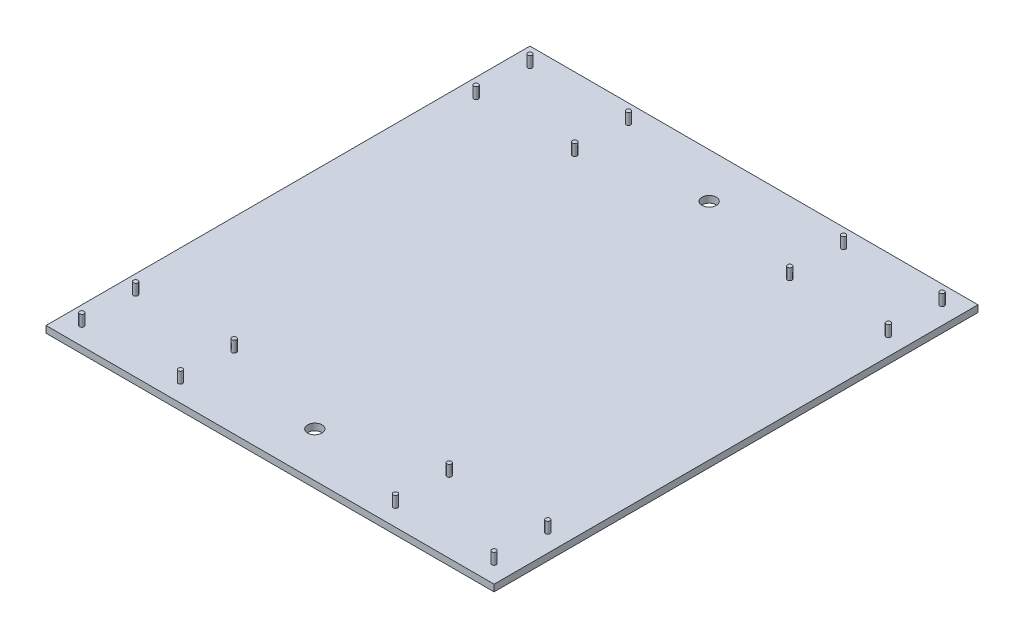
from build123d import *

# Parameters (mm, degrees)
SKETCH1_W           = 2000
SKETCH1_H           = 2160
BOSS_EXTRUDE1_DEPTH = 30
SKETCH2_R           = 10
BOSS_EXTRUDE2_DEPTH = 50
SKETCH3_R           = 32
CUT_EXTRUDE1_DEPTH  = 40


with BuildPart() as part:
    # Sketch1 → Boss-Extrude1 (new body)
    with BuildSketch(Plane(origin=(0, 0, 0), x_dir=(1, 0, 0), z_dir=(0, 1, 0))):
        Rectangle(SKETCH1_W, SKETCH1_H)
    extrude(amount=BOSS_EXTRUDE1_DEPTH)

    # Sketch2 → Boss-Extrude2 (add)
    with BuildSketch(Plane(origin=(0, 30, 0), x_dir=(1, 0, 0), z_dir=(0, 1, 0))):
        with Locations(Location((-920, 1000, 0), (0, 0, 90))):
            Circle(SKETCH2_R)
        with Locations(Location((-920, 760, 0), (0, 0, 90))):
            Circle(SKETCH2_R)
        with Locations(Location((-480, 1000, 0), (0, 0, 90))):
            Circle(SKETCH2_R)
        with Locations(Location((-480, 760, 0), (0, 0, 90))):
            Circle(SKETCH2_R)
        with Locations(Location((480, 760, 0), (0, 0, 90))):
            Circle(SKETCH2_R)
        with Locations(Location((480, 1000, 0), (0, 0, 90))):
            Circle(SKETCH2_R)
        with Locations(Location((920, 760, 0), (0, 0, 90))):
            Circle(SKETCH2_R)
        with Locations(Location((920, 1000, 0), (0, 0, 90))):
            Circle(SKETCH2_R)
        with Locations(Location((920, -1000, 0), (0, 0, 90))):
            Circle(SKETCH2_R)
        with Locations(Location((920, -760, 0), (0, 0, 90))):
            Circle(SKETCH2_R)
        with Locations(Location((480, -1000, 0), (0, 0, 90))):
            Circle(SKETCH2_R)
        with Locations(Location((480, -760, 0), (0, 0, 90))):
            Circle(SKETCH2_R)
        with Locations(Location((-480, -760, 0), (0, 0, 90))):
            Circle(SKETCH2_R)
        with Locations(Location((-480, -1000, 0), (0, 0, 90))):
            Circle(SKETCH2_R)
        with Locations(Location((-920, -760, 0), (0, 0, 90))):
            Circle(SKETCH2_R)
        with Locations(Location((-920, -1000, 0), (0, 0, 90))):
            Circle(SKETCH2_R)
    extrude(amount=BOSS_EXTRUDE2_DEPTH)

    # Sketch3 → Cut-Extrude1 (cut)
    with BuildSketch(Plane(origin=(0, 30, 0), x_dir=(1, 0, 0), z_dir=(0, 1, 0))):
        with Locations(Location((0, 880, 0), (0, 0, 270))):
            Circle(SKETCH3_R)
        with Locations(Location((0, -880, 0), (0, 0, 270))):
            Circle(SKETCH3_R)
    extrude(amount=-CUT_EXTRUDE1_DEPTH, mode=Mode.SUBTRACT)


solid = part.part
